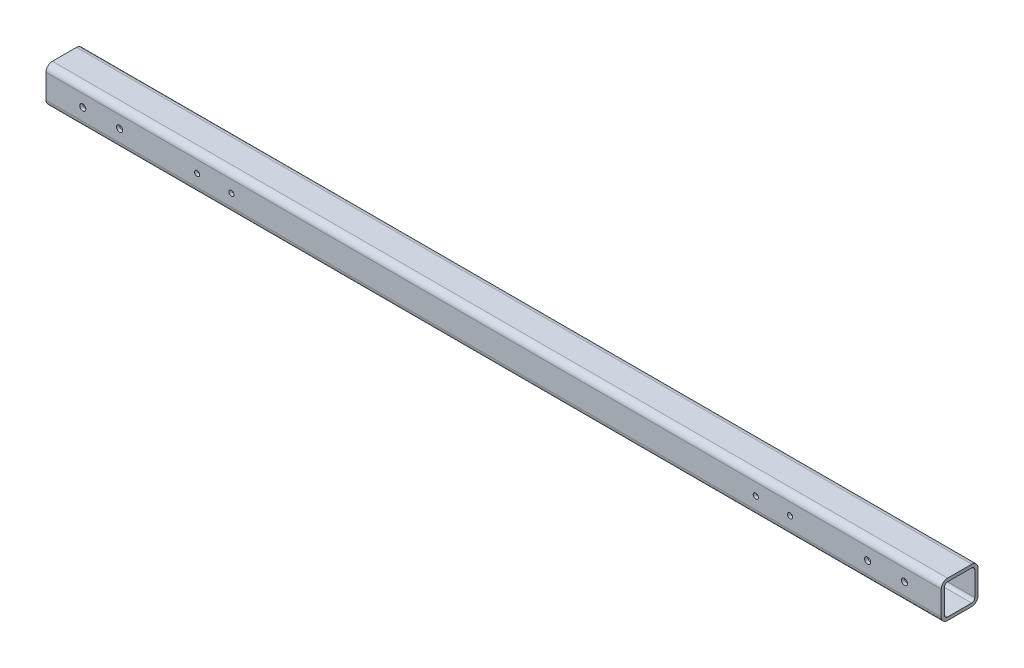
SolidWorks part; units mm, degrees
ref_plane "前视基准面" through (0, 0, 0) normal (0, 0, 1) x (1, 0, 0)
ref_plane "上视基准面" through (0, 0, 0) normal (0, 1, 0) x (1, 0, 0)
ref_plane "右视基准面" through (0, 0, 0) normal (1, 0, 0) x (0, 0, -1)
sketch3d "3D草图1"
  line L0 (0, 0, 0) -> (730, 0, 0)
  dimension "D1" = 730
other "结构构件1"
ref_plane "基准面1" through (0, 0, 0) normal (1, 0, 0) x (0, 0, -1)
sketch "Sketch1" plane through (0, 0, 0) normal (1, 0, 0) x (0, 0, -1)
  line L0 (-9.8, -12.4) -> (9.8, -12.4)
  line L1 (-12.4, -9.8) -> (-12.4, 9.8)
  line L2 (9.8, 12.4) -> (-9.8, 12.4)
  line L3 (12.4, 9.8) -> (12.4, -9.8)
  line L4 (-9.8, -15) -> (9.8, -15)
  line L5 (-15, -9.8) -> (-15, 9.8)
  line L6 (9.8, 15) -> (-9.8, 15)
  line L7 (15, 9.8) -> (15, -9.8)
  arc A0 (15, 9.8) -> (9.8, 15) centre (9.8, 9.8) ccw
  arc A1 (9.8, -15) -> (15, -9.8) centre (9.8, -9.8) ccw
  arc A2 (-15, -9.8) -> (-9.8, -15) centre (-9.8, -9.8) ccw
  arc A3 (-9.8, 15) -> (-15, 9.8) centre (-9.8, 9.8) ccw
  arc A4 (-9.8, 12.4) -> (-12.4, 9.8) centre (-9.8, 9.8) ccw
  arc A5 (12.4, 9.8) -> (9.8, 12.4) centre (9.8, 9.8) ccw
  arc A6 (9.8, -12.4) -> (12.4, -9.8) centre (9.8, -9.8) ccw
  arc A7 (-12.4, -9.8) -> (-9.8, -12.4) centre (-9.8, -9.8) ccw
  point P0 (-15, 0)
  point P1 (15, 0)
  point P2 (0, 15)
  point P3 (0, -15)
  point P4 (0, 0)
  point P5 (-15, -15)
  point P6 (15, -15)
  point P7 (15, 15)
  point P8 (-15, 15)
  point P33 (0, 0)
  dimension "D1" = 5.2
  dimension "Thickness" = 2.6
  dimension "V_leg" = 30
hole_wizard "M5 螺纹孔1" positions "草图2" profile "草图1" tap size "M5" standard "Iso" end condition through all
sketch "草图2" plane through (0, 0, 15) normal (0, 0, 1) x (1, 0, 0)
  line L0 (0, 9.8) -> (0, -9.8) construction
  line L1 (730, 9.8) -> (730, -9.8) construction
  point P0 (123.2, 0)
  point P5 (151.2, 0)
  point P8 (606.8, 0)
  point P10 (578.8, 0)
  dimension "D1" = 123.2
  dimension "D2" = 151.2
  dimension "D3" = 123.2
  dimension "D4" = 151.2
sketch "草图1" plane through (123.2, 0, 15) normal (1, 0, 0) x (0, -1, 0)
  line L0 (0, 0) -> (0, 30)
  line L1 (0, 30) -> (2.1, 30)
  line L2 (2.1, 30) -> (2.1, 0)
  line L5 (2.1, 0) -> (0, 0)
  line L11 (0, -6.35) -> (0, 107.95) construction
  dimension "通孔螺纹孔钻头直径" = 4.2
  dimension "通孔螺纹孔钻头深度" = 30
cosmetic thread "孔螺蚊线1" parameters "D2"=5
cosmetic thread "孔螺蚊线2" parameters "D2"=5
cosmetic thread "孔螺蚊线3" parameters "D2"=5
cosmetic thread "孔螺蚊线4" parameters "D2"=5
hole_wizard "M6 螺纹孔1" positions "草图4" profile "草图3" tap size "M6" standard "Iso" end condition through all
sketch "草图4" plane through (0, 0, 15) normal (0, 0, 1) x (1, 0, 0)
  line L0 (0, 9.8) -> (0, -9.8) construction
  line L1 (730, 9.8) -> (730, -9.8) construction
  point P0 (30, 0)
  point P2 (60, 0)
  point P4 (700, 0)
  point P6 (670, 0)
  dimension "D1" = 30
  dimension "D2" = 30
  dimension "D3" = 30
  dimension "D4" = 30
sketch "草图3" plane through (30, 0, 15) normal (1, 0, 0) x (0, -1, 0)
  line L0 (0, 0) -> (0, 30)
  line L1 (0, 30) -> (2.5, 30)
  line L2 (2.5, 30) -> (2.5, 0)
  line L5 (2.5, 0) -> (0, 0)
  line L11 (0, -6.35) -> (0, 107.95) construction
  dimension "通孔螺纹孔钻头直径" = 5
  dimension "通孔螺纹孔钻头深度" = 30
cosmetic thread "孔螺蚊线5" parameters "D2"=6
cosmetic thread "孔螺蚊线6" parameters "D2"=6
cosmetic thread "孔螺蚊线7" parameters "D2"=6
cosmetic thread "孔螺蚊线8" parameters "D2"=6
